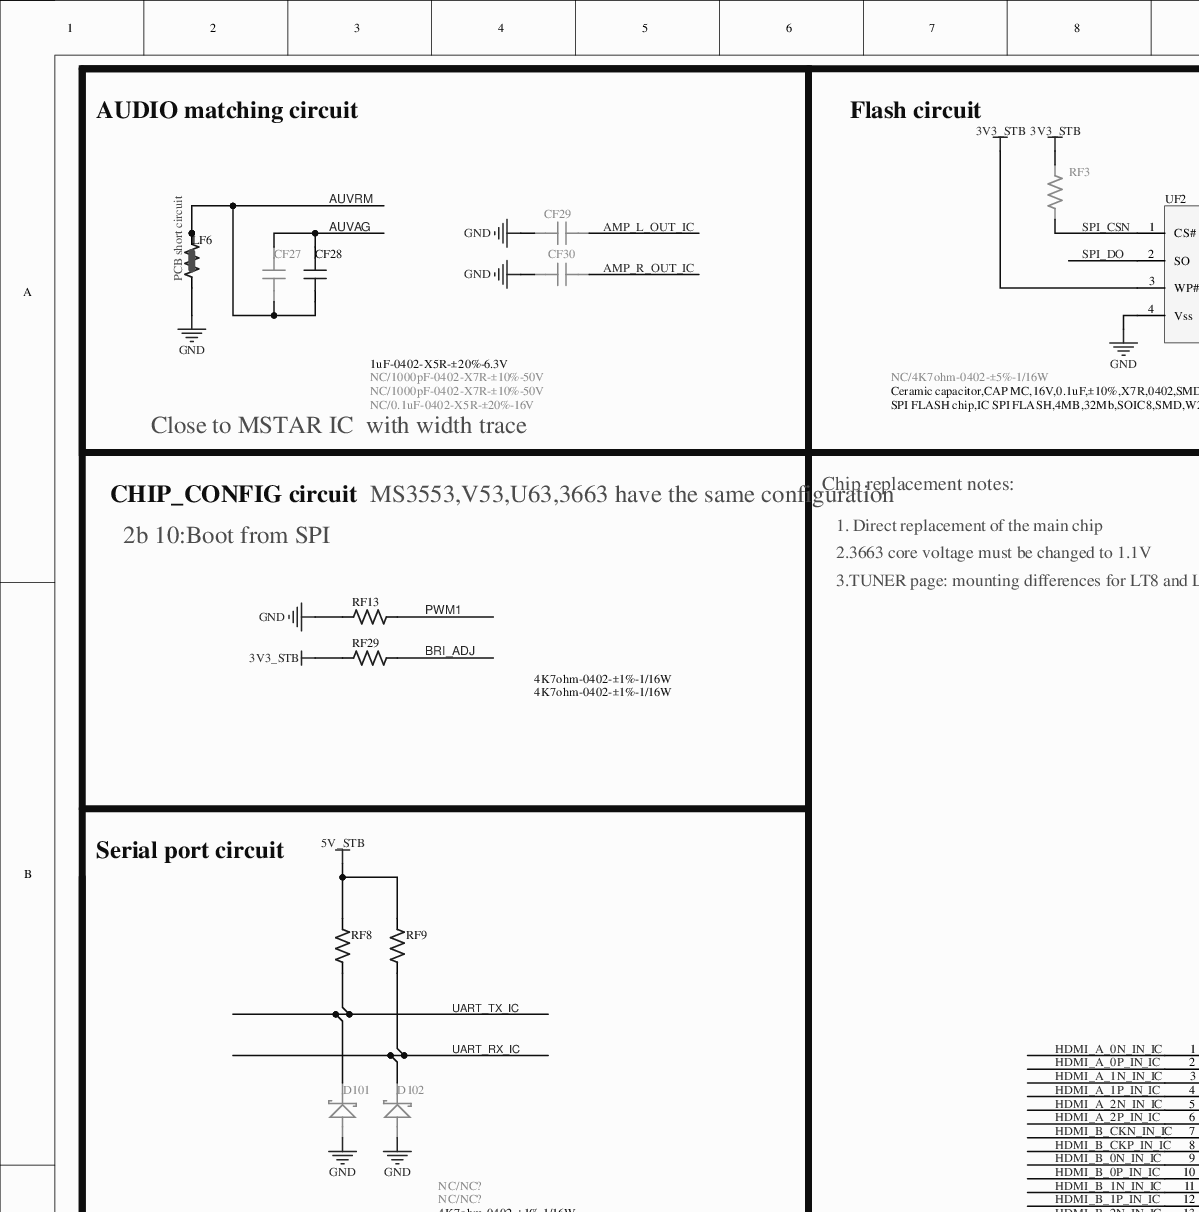
[diagram p0: MISC116569-7.SchDoc, top left]
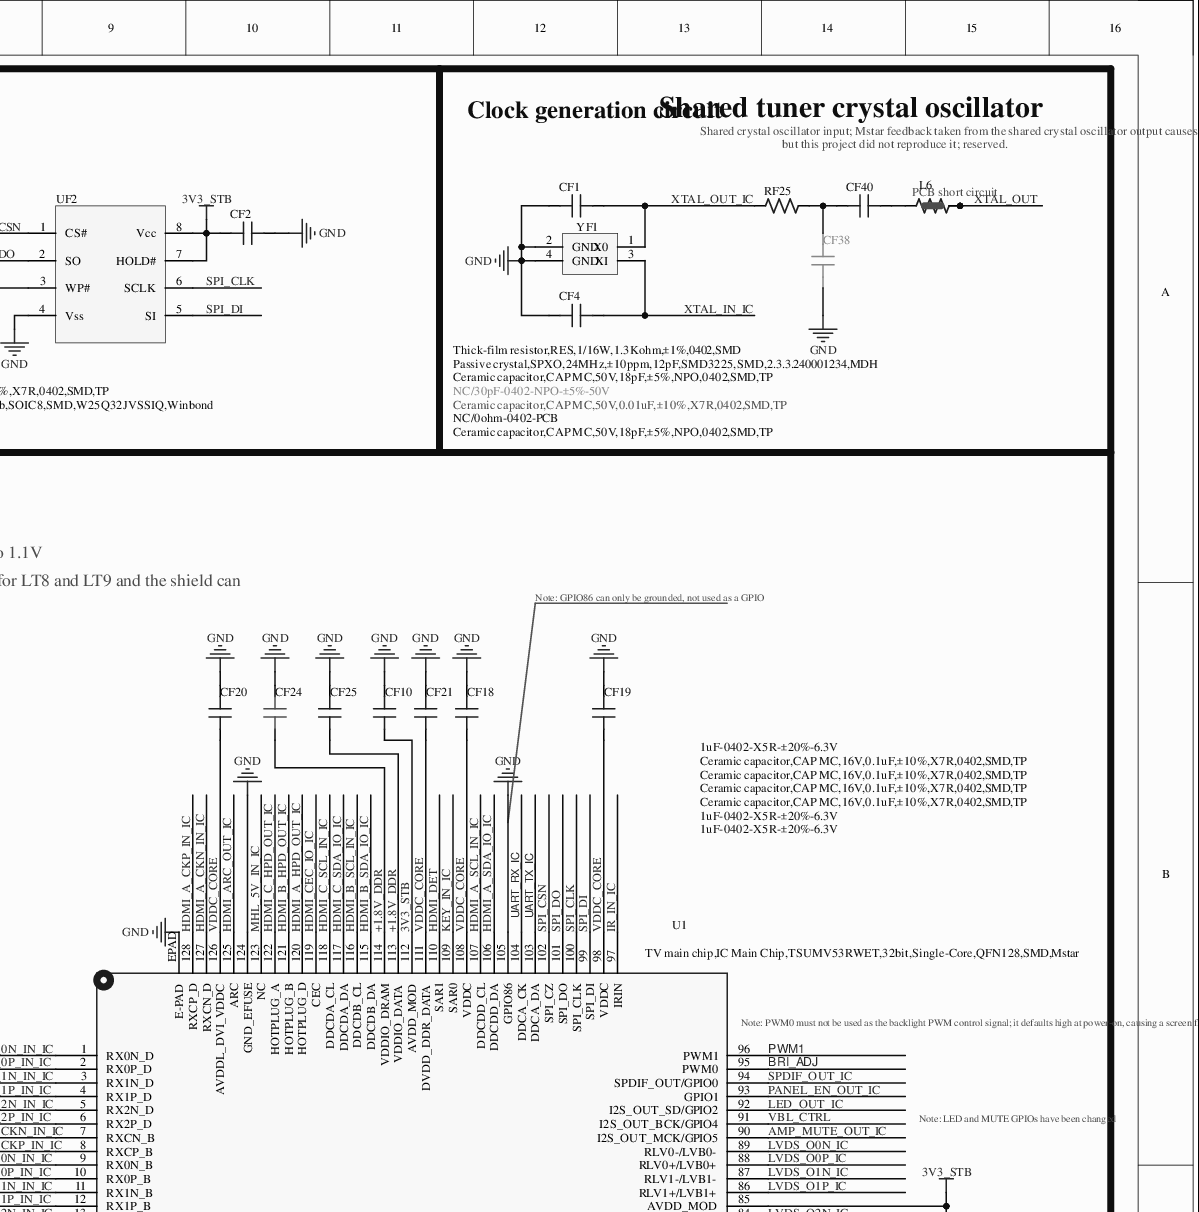
[diagram p1: MISC116569-7.SchDoc, top right]
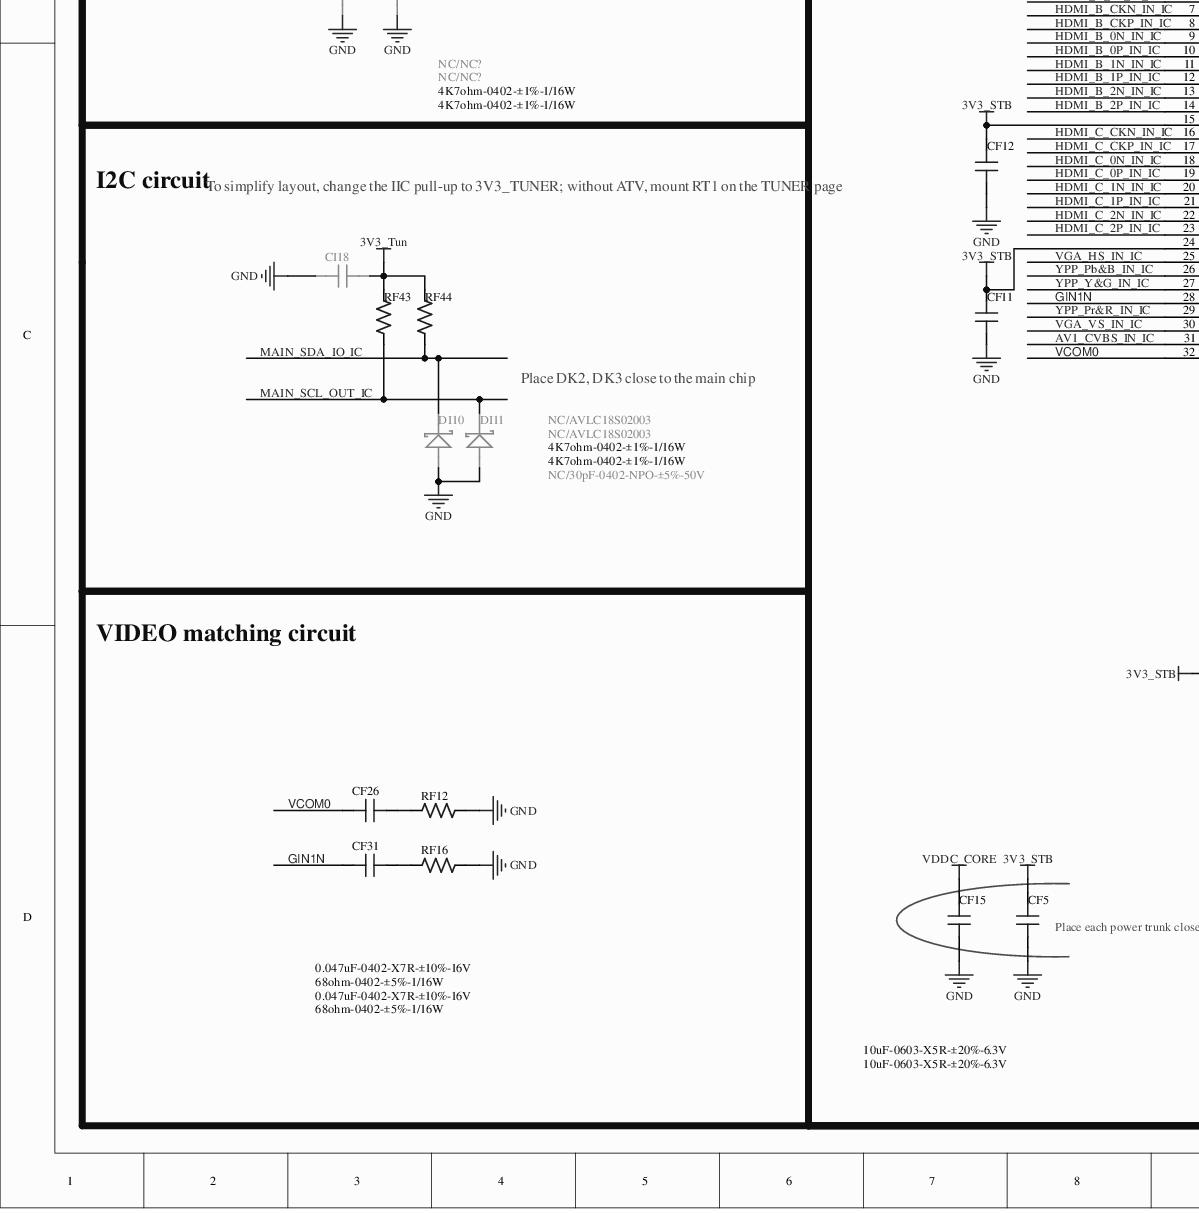
[diagram p2: MISC116569-7.SchDoc, bottom left]
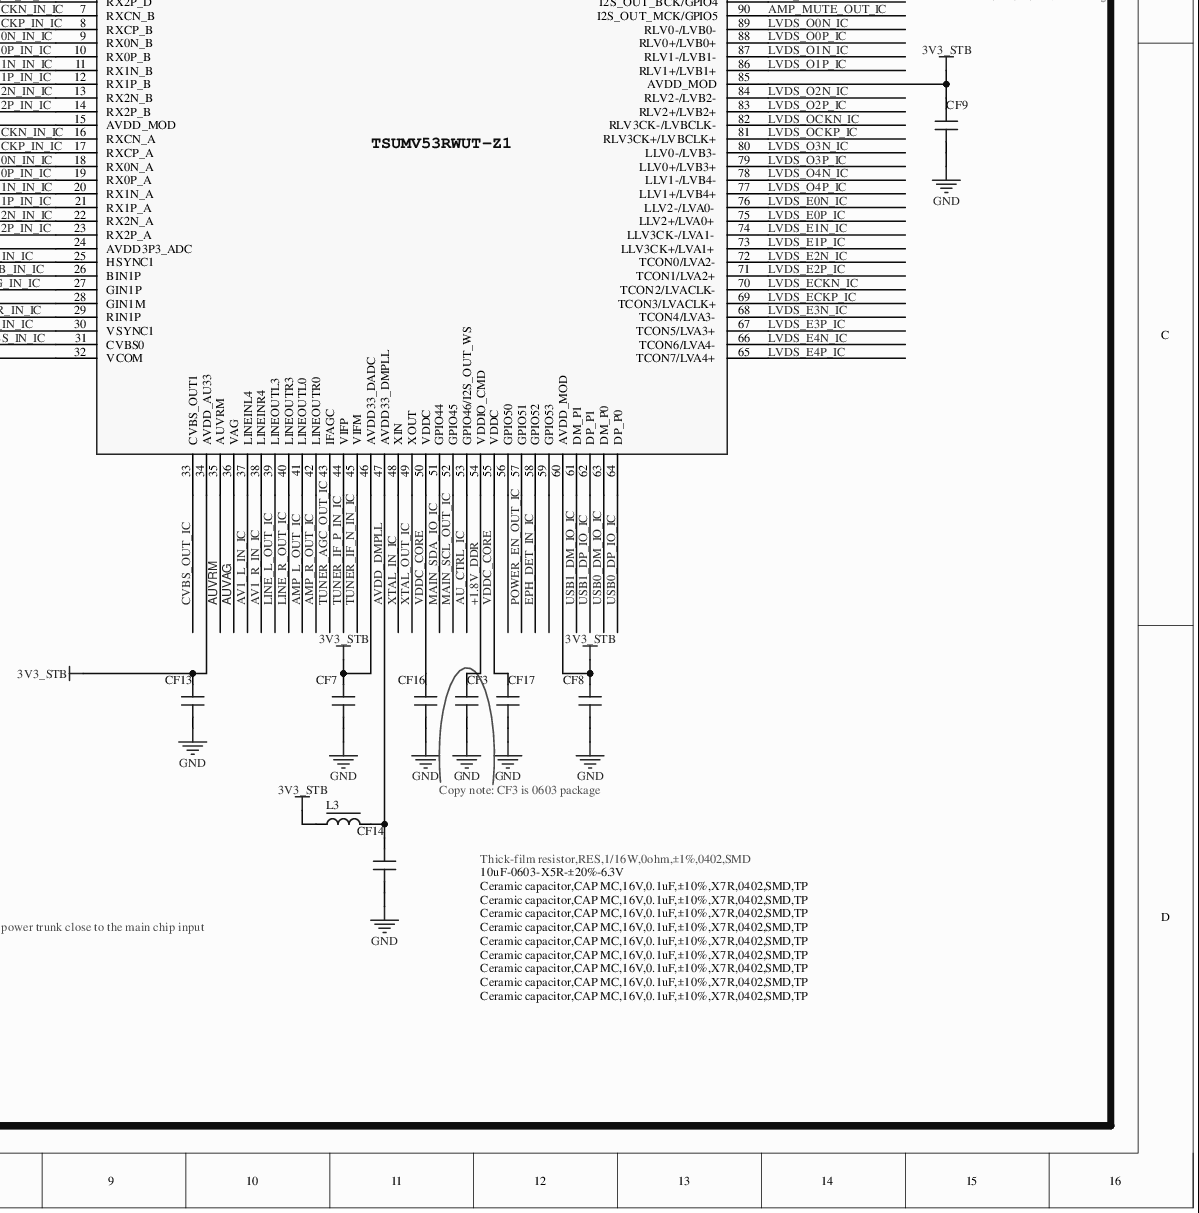
[diagram p3: MISC116569-7.SchDoc, bottom right]
# Altium project MISC116569-15.PrjPCB (part 3 of 8)

## Sheet MISC116569-7.SchDoc
size 426 x 431 mm

### Parts
CF1  Ceramic capacitor,CAP MC,50V,18pF,±5%,NPO,0402,SMD,TP  [C0402]
CF2  Ceramic capacitor,CAP MC,16V,0.1uF,±10%,X7R,0402,SMD,TP  [C0402]
CF3  10uF-0603-X5R-±20%-6.3V  [C0603]
CF4  Ceramic capacitor,CAP MC,50V,18pF,±5%,NPO,0402,SMD,TP  [C0402]
CF5  10uF-0603-X5R-±20%-6.3V  [C0603]
CF7  Ceramic capacitor,CAP MC,16V,0.1uF,±10%,X7R,0402,SMD,TP  [C0402]
CF8  Ceramic capacitor,CAP MC,16V,0.1uF,±10%,X7R,0402,SMD,TP  [C0402]
CF9  Ceramic capacitor,CAP MC,16V,0.1uF,±10%,X7R,0402,SMD,TP  [C0402]
CF10  Ceramic capacitor,CAP MC,16V,0.1uF,±10%,X7R,0402,SMD,TP  [C0402]
CF11  Ceramic capacitor,CAP MC,16V,0.1uF,±10%,X7R,0402,SMD,TP  [C0402]
CF12  Ceramic capacitor,CAP MC,16V,0.1uF,±10%,X7R,0402,SMD,TP  [C0402]
CF13  Ceramic capacitor,CAP MC,16V,0.1uF,±10%,X7R,0402,SMD,TP  [C0402]
CF14  Ceramic capacitor,CAP MC,16V,0.1uF,±10%,X7R,0402,SMD,TP  [C0402]
CF15  10uF-0603-X5R-±20%-6.3V  [C0603]
CF16  Ceramic capacitor,CAP MC,16V,0.1uF,±10%,X7R,0402,SMD,TP  [C0402]
CF17  Ceramic capacitor,CAP MC,16V,0.1uF,±10%,X7R,0402,SMD,TP  [C0402]
CF18  Ceramic capacitor,CAP MC,16V,0.1uF,±10%,X7R,0402,SMD,TP  [C0402]
CF19  Ceramic capacitor,CAP MC,16V,0.1uF,±10%,X7R,0402,SMD,TP  [C0402]
CF20  Ceramic capacitor,CAP MC,16V,0.1uF,±10%,X7R,0402,SMD,TP  [C0402]
CF21  1uF-0402-X5R-±20%-6.3V  [C0402]
CF24  1uF-0402-X5R-±20%-6.3V  [C0402]
CF25  1uF-0402-X5R-±20%-6.3V  [C0402]
CF26  0.047uF-0402-X7R-±10%-16V  [C0402]
CF27  NC/0.1uF-0402-X5R-±20%-16V  [C0402]
CF28  1uF-0402-X5R-±20%-6.3V  [C0402]
CF29  NC/1000pF-0402-X7R-±10%-50V  [C0402]
CF30  NC/1000pF-0402-X7R-±10%-50V  [C0402]
CF31  0.047uF-0402-X7R-±10%-16V  [C0402]
CF38  NC/30pF-0402-NPO-±5%-50V  [C0402]
CF40  Ceramic capacitor,CAP MC,50V,0.01uF,±10%,X7R,0402,SMD,TP  [C0402]
CI18  NC/30pF-0402-NPO-±5%-50V  [C0402]
D101  NC/NC?  [DIODE-S0402]
D102  NC/NC?  [DIODE-S0402]
DI10  NC/AVLC18S02003  [DIODE-S0402]
DI11  NC/AVLC18S02003  [DIODE-S0402]
L3  Thick-film resistor,RES,1/16W,0ohm,±1%,0402,SMD  [L0402]
L6  NC/0ohm-0402-PCB  [R0402SC]
LF6  NC/0ohm-0402-PCB  [R0402SC]  (value not drawn)
RF3  NC/4K7ohm-0402-±5%-1/16W  [R0402]
RF8  4K7ohm-0402-±1%-1/16W  [R0402]
RF9  4K7ohm-0402-±1%-1/16W  [R0402]
RF12  68ohm-0402-±5%-1/16W  [R0402]
RF13  4K7ohm-0402-±1%-1/16W  [R0402]
RF16  68ohm-0402-±5%-1/16W  [R0402]
RF25  Thick-film resistor,RES,1/16W,1.3Kohm,±1%,0402,SMD  [R0402]
RF29  4K7ohm-0402-±1%-1/16W  [R0402]
RF43  4K7ohm-0402-±1%-1/16W  [R0402]
RF44  4K7ohm-0402-±1%-1/16W  [R0402]
U1  TV main chip,IC Main Chip,TSUMV53RWET,32bit,Single-Core,QFN128,SMD,Mstar  [QFN128/0.35-1]
UF2  SPI FLASH chip,IC SPI FLASH,4MB,32Mb,SOIC8,SMD,W25Q32JVSSIQ,Winbond  [SOIC8]
YF1  Passive crystal,SPXO,24MHz,±10ppm,12pF,SMD3225,SMD,2.3.3.240001234,MDH  [XTAL-S-3]

### Blocks framed on the sheet
Flash circuit: CF2 RF3 UF2
VIDEO matching circuit: CF26 CF31 RF12 RF16

### Nets
3V3_STB: CF2.2 CF5.2 CF7.2 CF8.2 CF9.2 CF10.2 CF11.1 CF12.2 CF13.2 L3.1 RF3.2 RF29.2 U1.15(AVDD_MOD) U1.24(AVDD3P3_ADC) U1.34(AVDD_AU33) U1.46(AVDD33_DADC) U1.60(AVDD_MOD) U1.85(AVDD_MOD) U1.112(AVDD_MOD) UF2.3(WP#) UF2.7(HOLD#) UF2.8(Vcc)
3V3_Tun: CI18.2 RF43.1 RF44.1
5V_STB: RF8.2 RF9.2
+1.8V_DDR: CF3.2 CF24.1 CF25.1 U1.54(VDDIO_CMD) U1.113(VDDIO_DATA) U1.114(VDDIO_DRAM)
GND: CF1.1 CF2.1 CF3.1 CF4.1 CF5.1 CF7.1 CF8.1 CF9.1 CF10.1 CF11.2 CF12.1 CF13.1 CF14.1 CF15.1 CF16.1 CF17.1 CF18.2 CF19.2 CF20.1 CF21.2 CF24.2 CF25.2 CF29.2 CF30.2 CF38.1 CI18.1 D101.A D102.A DI10.A DI11.A LF6.1 RF12.2 RF13.2 RF16.2 U1.105(GPIO86) U1.124(GND_EFUSE) U1.EPAD(E-PAD) UF2.4(Vss) YF1.2(GND) YF1.4(GND)
VDDC_CORE: CF15.2 CF16.2 CF17.2 CF18.1 CF19.1 CF20.2 CF21.1 U1.50(VDDC) U1.55(VDDC) U1.98(VDDC) U1.108(VDDC) U1.111(DVDD_DDR_DATA) U1.126(AVDDL_DVI_VDDC)
AMP_L_OUT_IC: CF29.1 U1.41(LINEOUTL0)
AMP_MUTE_OUT_IC: U1.90(I2S_OUT_MCK/GPIO5)
AMP_R_OUT_IC: CF30.1 U1.42(LINEOUTR0)
AU_CTRL_IC: U1.53(GPIO46/I2S_OUT_WS)
AUVAG: CF27.2 CF28.2 U1.36(VAG)
AUVRM: CF27.1 CF28.1 LF6.2 LF6.3 U1.35(AUVRM)
AV1_CVBS_IN_IC: U1.31(CVBS0)
AV1_L_IN_IC: U1.37(LINEINL4)
AV1_R_IN_IC: U1.38(LINEINR4)
AVDD_DMPLL: CF14.2 L3.2 U1.47(AVDD33_DMPLL)
BRI_ADJ: RF29.1 U1.95(PWM0)
CVBS_OUT_IC: U1.33(CVBS_OUT1)
EPH_DET_IN_IC: U1.58(GPIO52)
GIN1N: CF31.1 U1.28(GIN1M)
HDMI_A_0N_IN_IC: U1.1(RX0N_D)
HDMI_A_0P_IN_IC: U1.2(RX0P_D)
HDMI_A_1N_IN_IC: U1.3(RX1N_D)
HDMI_A_1P_IN_IC: U1.4(RX1P_D)
HDMI_A_2N_IN_IC: U1.5(RX2N_D)
HDMI_A_2P_IN_IC: U1.6(RX2P_D)
HDMI_A_CKN_IN_IC: U1.127(RXCN_D)
HDMI_A_CKP_IN_IC: U1.128(RXCP_D)
HDMI_A_HPD_OUT_IC: U1.120(HOTPLUG_D)
HDMI_A_SCL_IN_IC: U1.107(DDCDD_CL)
HDMI_A_SDA_IO_IC: U1.106(DDCDD_DA)
HDMI_ARC_OUT_IC: U1.125(ARC)
HDMI_B_0N_IN_IC: U1.9(RX0N_B)
HDMI_B_0P_IN_IC: U1.10(RX0P_B)
HDMI_B_1N_IN_IC: U1.11(RX1N_B)
HDMI_B_1P_IN_IC: U1.12(RX1P_B)
HDMI_B_2N_IN_IC: U1.13(RX2N_B)
HDMI_B_2P_IN_IC: U1.14(RX2P_B)
HDMI_B_CKN_IN_IC: U1.7(RXCN_B)
HDMI_B_CKP_IN_IC: U1.8(RXCP_B)
HDMI_B_HPD_OUT_IC: U1.121(HOTPLUG_B)
HDMI_B_SCL_IN_IC: U1.116(DDCDB_CL)
HDMI_B_SDA_IO_IC: U1.115(DDCDB_DA)
HDMI_C_0N_IN_IC: U1.18(RX0N_A)
HDMI_C_0P_IN_IC: U1.19(RX0P_A)
HDMI_C_1N_IN_IC: U1.20(RX1N_A)
HDMI_C_1P_IN_IC: U1.21(RX1P_A)
HDMI_C_2N_IN_IC: U1.22(RX2N_A)
HDMI_C_2P_IN_IC: U1.23(RX2P_A)
HDMI_C_CKN_IN_IC: U1.16(RXCN_A)
HDMI_C_CKP_IN_IC: U1.17(RXCP_A)
HDMI_C_HPD_OUT_IC: U1.122(HOTPLUG_A)
HDMI_C_SCL_IN_IC: U1.118(DDCDA_CL)
HDMI_C_SDA_IO_IC: U1.117(DDCDA_DA)
HDMI_CEC_IO_IC: U1.119(CEC)
HDMI_DET: U1.110(SAR1)
IR_IN_IC: U1.97(IRIN)
KEY_IN_IC: U1.109(SAR0)
LED_OUT_IC: U1.92(I2S_OUT_SD/GPIO2)
LINE_L_OUT_IC: U1.39(LINEOUTL3)
LINE_R_OUT_IC: U1.40(LINEOUTR3)
LVDS_E0N_IC: U1.76(LLV2-/LVA0-)
LVDS_E0P_IC: U1.75(LLV2+/LVA0+)
LVDS_E1N_IC: U1.74(LLV3CK-/LVA1-)
LVDS_E1P_IC: U1.73(LLV3CK+/LVA1+)
LVDS_E2N_IC: U1.72(TCON0/LVA2-)
LVDS_E2P_IC: U1.71(TCON1/LVA2+)
LVDS_E3N_IC: U1.68(TCON4/LVA3-)
LVDS_E3P_IC: U1.67(TCON5/LVA3+)
LVDS_E4N_IC: U1.66(TCON6/LVA4-)
LVDS_E4P_IC: U1.65(TCON7/LVA4+)
LVDS_ECKN_IC: U1.70(TCON2/LVACLK-)
LVDS_ECKP_IC: U1.69(TCON3/LVACLK+)
LVDS_O0N_IC: U1.89(RLV0-/LVB0-)
LVDS_O0P_IC: U1.88(RLV0+/LVB0+)
LVDS_O1N_IC: U1.87(RLV1-/LVB1-)
LVDS_O1P_IC: U1.86(RLV1+/LVB1+)
LVDS_O2N_IC: U1.84(RLV2-/LVB2-)
LVDS_O2P_IC: U1.83(RLV2+/LVB2+)
LVDS_O3N_IC: U1.80(LLV0-/LVB3-)
LVDS_O3P_IC: U1.79(LLV0+/LVB3+)
LVDS_O4N_IC: U1.78(LLV1-/LVB4-)
LVDS_O4P_IC: U1.77(LLV1+/LVB4+)
LVDS_OCKN_IC: U1.82(RLV3CK-/LVBCLK-)
LVDS_OCKP_IC: U1.81(RLV3CK+/LVBCLK+)
MAIN_SCL_OUT_IC: DI11.K RF43.2 U1.52(GPIO45)
MAIN_SDA_IO_IC: DI10.K RF44.2 U1.51(GPIO44)
MHL_5V_IN_IC: U1.123(NC)
PANEL_EN_OUT_IC: U1.93(GPIO1)
POWER_EN_OUT_IC: U1.57(GPIO51)
PWM1: RF13.1 U1.96(PWM1)
SPDIF_OUT_IC: U1.94(SPDIF_OUT/GPIO0)
SPI_CLK: U1.100(SPI_CLK) UF2.6(SCLK)
SPI_CSN: RF3.1 U1.102(SPI_CZ) UF2.1(CS#)
SPI_DI: U1.99(SPI_DI) UF2.5(SI)
SPI_DO: U1.101(SPI_DO) UF2.2(SO)
TUNER_AGC_OUT_IC: U1.43(IFAGC)
TUNER_IF_N_IN_IC: U1.45(VIFM)
TUNER_IF_P_IN_IC: U1.44(VIFP)
UART_RX_IC: D102.K RF9.1 U1.104(DDCA_CK)
UART_TX_IC: D101.K RF8.1 U1.103(DDCA_DA)
USB0_DM_IO_IC: U1.63(DM_P0)
USB0_DP_IO_IC: U1.64(DP_P0)
USB1_DM_IO_IC: U1.61(DM_P1)
USB1_DP_IO_IC: U1.62(DP_P1)
VBL_CTRL: U1.91(I2S_OUT_BCK/GPIO4)
VCOM0: CF26.1 U1.32(VCOM)
VGA_HS_IN_IC: U1.25(HSYNC1)
VGA_VS_IN_IC: U1.30(VSYNC1)
XTAL_IN_IC: CF4.2 U1.48(XIN) YF1.3(XI)
XTAL_OUT: L6.2 L6.3
XTAL_OUT_IC: CF1.2 RF25.2 U1.49(XOUT) YF1.1(X0)
YPP_Pb&B_IN_IC: U1.26(BIN1P)
YPP_Pr&R_IN_IC: U1.29(RIN1P)
YPP_Y&G_IN_IC: U1.27(GIN1P)
NetCF26_2: CF26.2 RF12.1
NetCF31_2: CF31.2 RF16.1
NetCF38_2: CF38.2 CF40.2 RF25.1
NetCF40_1: CF40.1 L6.1

Not connected (* = marked no-connect by the designer): U1 56(GPIO50)* 59(GPIO53)*

### Notes on the sheet
- AUDIO matching circuit
- Clock generation circuit
- Shared tuner crystal oscillator
- Shared crystal oscillator input; Mstar feedback taken from the shared crystal oscillator output causes DVB_T2/C issues,
- but this project did not reproduce it; reserved.
- Close to MSTAR IC  with width trace
- CHIP_CONFIG circuit
- MS3553,V53,U63,3663 have the same configuration
- Chip replacement notes:
- 2b 10:Boot from SPI
- 1. Direct replacement of the main chip
- 2.3663 core voltage must be changed to 1.1V
- 3.TUNER page: mounting differences for LT8 and LT9 and the shield can
- Note: GPIO86 can only be grounded, not used as a GPIO
- Serial port circuit
- (near U1) Note: PWM0 must not be used as the backlight PWM control signal; it defaults high at power-on, causing a screen flash
- Note: LED and MUTE GPIOs have been changed
- I2C circuit
- To simplify layout, change the IIC pull-up to 3V3_TUNER; without ATV, mount RT1 on the TUNER page
- Place DK2, DK3 close to the main chip
- Copy note: CF3 is 0603 package
- (near CF5) Place each power trunk close to the main chip input

### Library data of the parts
CF1 CF4 = 004.003.0000527-D: Ceramic capacitor,CAP MC,50V,18pF,±5%,NPO,0402,SMD,TP-D
CF2 CF7-CF10 CF12-CF14 CF17 CF27 = 0.1uF-0402-Y5V-+80%-20%-16V-D
CF3 CF5 CF15 = 10uF-0603-X5R-±20%-6.3V-D
CF11 CF16 CF18-CF21 CF25 CF28 = 1uF-0402-X5R-±20%-6.3V-D
CF24 = 004.003.0000100-D: Ceramic capacitor,CAP MC,6.3V,2.2uF,±20%,X5R,0402,SMD,TP-D
CF26 CF31 = 0.047uF-0402-X7R-±10%-16V-D
CF29 CF30 = 1000pF-0402-X7R-±10%-50V-D
CF38 CF40 CI18 = 30pF-0402-NPO-±5%-50V-D
D101 D102 DI10 DI11 = AVLC18S02003-D
L3 = FCM1005KF-121T06(120ohm-500mA)-D
L6 LF6 = 0ohm-0402-PCB-D
RF3 RF8 RF9 RF13 RF29 RF43 RF44 = 4K7ohm-0402-±5%-1/16W-D
RF12 RF16 = 68ohm-0402-±5%-1/16W-D
RF25 = 1Kohm-0402-±5%-1/16W-D
U1 = 004.016.0001146-D: TV main chip,IC Main Chip,TSUMV53RWUT-Z1,32bit,Single-Core,QFN128,SMD,Mstar-D
UF2 = SPI FLASH 芯片,IC SPI FLASH,32Mb,SOIC8,SMD,GD25Q32CSIG,GigaDevice-D
YF1 = 16.000MHz±20PPM-10PF-SMD3225-D: NC: GPS; PCB DECAL: TCXO_3225; Source_Path: EM_66_V2.0_201209181010.DSN; Value: 26M/0.5PPM/1.8V